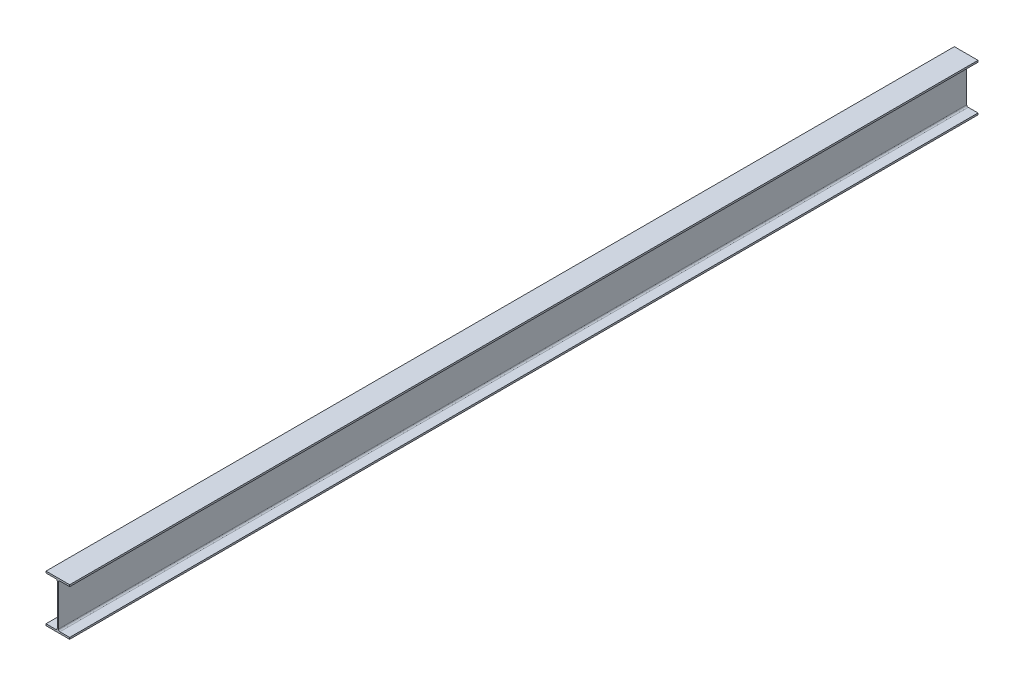
from build123d import *

# Parameters (mm, degrees)
BOSS_EXTRUDE1_DEPTH = 4800


with BuildPart() as part:
    # Sketch1 → Boss-Extrude1 (new body)
    with BuildSketch(Plane.XY):
        with BuildLine():
            Line((62.5, 0), (-62.5, 0))
            Line((-62.5, 0), (-62.5, 9))
            Line((-62.5, 9), (-11, 9))
            ThreePointArc((-11, 9), (-5.343145751, 11.343145751), (-3, 17))
            Line((-3, 17), (-3, 233))
            ThreePointArc((-3, 233), (-5.343145751, 238.656854249), (-11, 241))
            Line((-11, 241), (-62.5, 241))
            Line((-62.5, 241), (-62.5, 250))
            Line((-62.5, 250), (62.5, 250))
            Line((62.5, 250), (62.5, 241))
            Line((62.5, 241), (11, 241))
            ThreePointArc((11, 241), (5.343145751, 238.656854249), (3, 233))
            Line((3, 233), (3, 17))
            ThreePointArc((3, 17), (5.343145751, 11.343145751), (11, 9))
            Line((11, 9), (62.5, 9))
            Line((62.5, 9), (62.5, 0))
        make_face()
    extrude(amount=BOSS_EXTRUDE1_DEPTH)


solid = part.part
